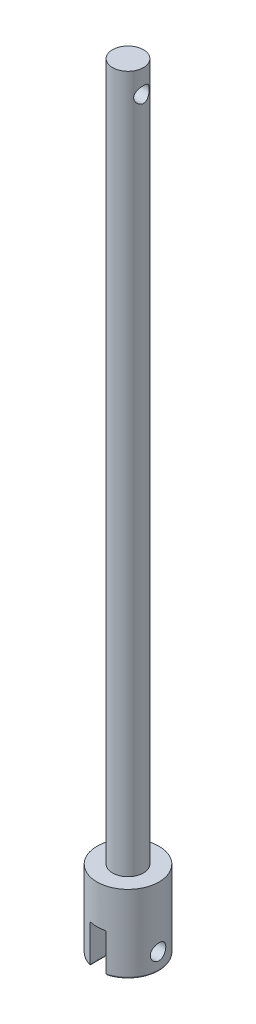
SolidWorks part; units mm, degrees
material "1.7005 (45Cr2)"
ref_plane "前视基准面" through (0, 0, 0) normal (0, 0, 1) x (1, 0, 0)
ref_plane "上视基准面" through (0, 0, 0) normal (0, 1, 0) x (1, 0, 0)
ref_plane "右视基准面" through (0, 0, 0) normal (1, 0, 0) x (0, 0, -1)
sketch "草图11" plane through (0, 0, 0) normal (0, -1, 0) x (1, 0, 0)
  circle A0 centre (0, 0) radius 2
  dimension "D1" = 4
extrude "凸台-拉伸3" add sketch "草图11" along normal blind 100
sketch "草图20" plane through (0, -100, 0) normal (0, -1, 0) x (1, 0, 0)
  circle A2 centre (0, 0) radius 4
  circle A3 centre (0, 0) radius 4
  dimension "D1" = 2
extrude "凸台-拉伸4" add sketch "草图20" against normal blind 10
sketch "草图16" plane through (0, 0, 0) normal (0, 0, 1) x (1, 0, 0)
  line L5 (-2, -100) -> (2, -100) construction
  line L6 (1.05, -95) -> (-1.05, -95)
  line L12 (1.05, -95) -> (1.05, -100)
  line L13 (1.05, -100) -> (-1.05, -100)
  line L15 (-1.05, -95) -> (-1.05, -100)
  line L16 (1.05, -95) -> (-1.05, -100) construction
  line L17 (1.05, -100) -> (-1.05, -95) construction
  line L18 (0, -97.5) -> (0, -100) construction
  point P0 (0, -97.5)
  dimension "D1" = 2.1
  dimension "D2" = 5
extrude "切除-拉伸5" cut sketch "草图16" against normal mid plane 400
sketch "草图18" plane through (-1.05, 0, 0) normal (1, 0, 0) x (0, 0, -1)
  line L0 (-2, -90) -> (2, -90) construction
  line L2 (0, -97.8) -> (0, -100) construction
  line L3 (-1.7022, -100) -> (1.7022, -100) construction
  circle A0 centre (0, -97.8) radius 1
  dimension "D1" = 2
  dimension "D2" = 2.2
extrude "切除-拉伸7" cut sketch "草图18" against normal mid plane 400
sketch "草图19" plane through (0, 0, 0) normal (1, 0, 0) x (0, 0, -1)
  line L0 (2, 0) -> (-2, 0) construction
  line L1 (0, 0) -> (0, -3) construction
  circle A0 centre (0, -3) radius 1
  dimension "D1" = 2
  dimension "D2" = 3
extrude "切除-拉伸8" cut sketch "草图19" against normal mid plane 10
fillet "圆角1" radius 0.2 4 edges at (1.05, -100, 0) (-1.05, -100, 0) (4, -100, 0) (-4, -100, 0)
fillet "圆角2" radius 0.2 2 edges at (-1.05, -95, 0) (1.05, -95, 0)
